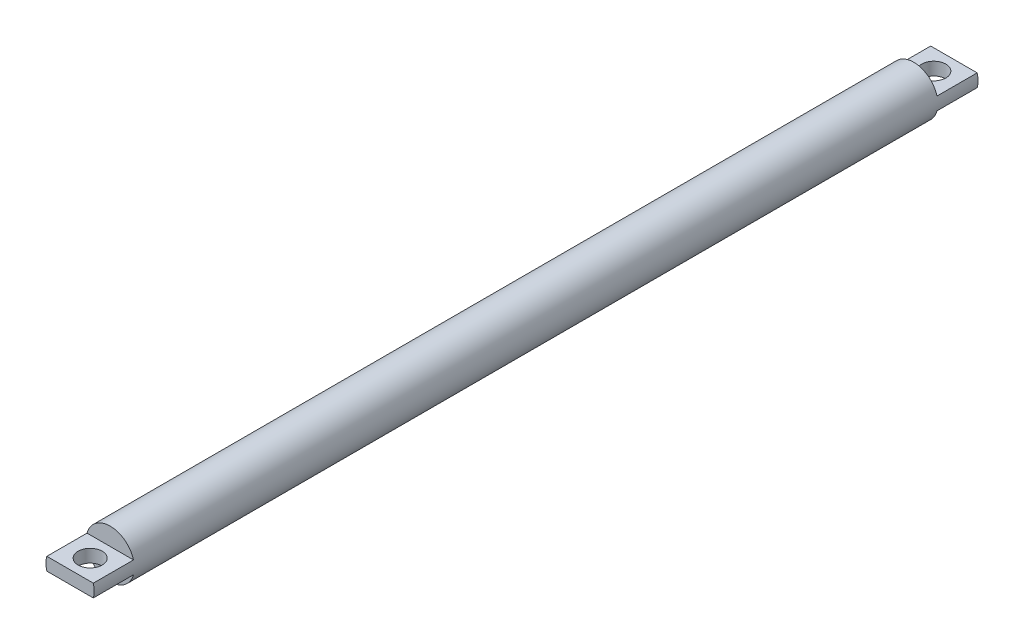
SolidWorks part; units mm, degrees
ref_plane "前视基准面" through (0, 0, 0) normal (0, 0, 1) x (1, 0, 0)
ref_plane "上视基准面" through (0, 0, 0) normal (0, 1, 0) x (1, 0, 0)
ref_plane "右视基准面" through (0, 0, 0) normal (1, 0, 0) x (0, 0, -1)
other "Configuration Table"
sketch "草图1" plane through (0, 0, 0) normal (0, 0, 1) x (1, 0, 0)
  circle A0 centre (0, 0) radius 3
extrude "凸台-拉伸1" add sketch "草图1" along normal blind 100
sketch "草图2" plane through (0, 0, 100) normal (0, 0, 1) x (1, 0, 0)
  line L0 (-4.1691, 0) -> (4.4307, 0) construction
  line L1 (-2.8914, 0.8) -> (2.8914, 0.8)
  line L2 (-2.8914, -0.8) -> (2.8914, -0.8)
  circle A0 centre (0, 0) radius 3 construction
  arc A1 (2.8914, -0.8) -> (2.8914, 0.8) centre (0, 0) ccw
  arc A2 (-2.8914, 0.8) -> (-2.8914, -0.8) centre (0, 0) ccw
  dimension "D1" = 0.8
extrude "凸台-拉伸3" add sketch "草图2" along normal blind 5
sketch "草图8" plane through (0, 0, 0) normal (0, 0, -1) x (-1, 0, 0)
  line L0 (-2.8914, 0.8) -> (2.8914, 0.8)
  line L1 (-2.8914, -0.8) -> (2.8914, -0.8)
  line L2 (-4.1024, 0) -> (4.2031, 0) construction
  arc A1 (-2.8914, 0.8) -> (-2.8914, -0.8) centre (0, 0) ccw
  arc A2 (2.8914, -0.8) -> (2.8914, 0.8) centre (0, 0) ccw
extrude "凸台-拉伸4" add sketch "草图8" along normal blind 5
sketch "草图9" plane through (0, 0.8, 0) normal (0, 1, 0) x (1, 0, 0)
  line L0 (0, 6.0875) -> (0, -1.2478) construction
  line L1 (-5.7998, 2.5) -> (5.9634, 2.5) construction
  line L2 (-2.8914, 5) -> (2.8914, 5) construction
  circle A0 centre (0, 2.5) radius 1.5
  dimension "D1" = 2.5
extrude "切除-拉伸1" cut sketch "草图9" against normal blind 5
sketch "草图10" plane through (0, 0.8, 0) normal (0, 1, 0) x (1, 0, 0)
  line L0 (0, -98.7619) -> (0, -105.4166) construction
  line L1 (-5.0462, -102.5) -> (6.7181, -102.5) construction
  line L2 (2.8914, -105) -> (-2.8914, -105) construction
  circle A0 centre (0, -102.5) radius 1.5
  dimension "D1" = 2.5
extrude "切除-拉伸2" cut sketch "草图10" against normal blind 5 contours A0
